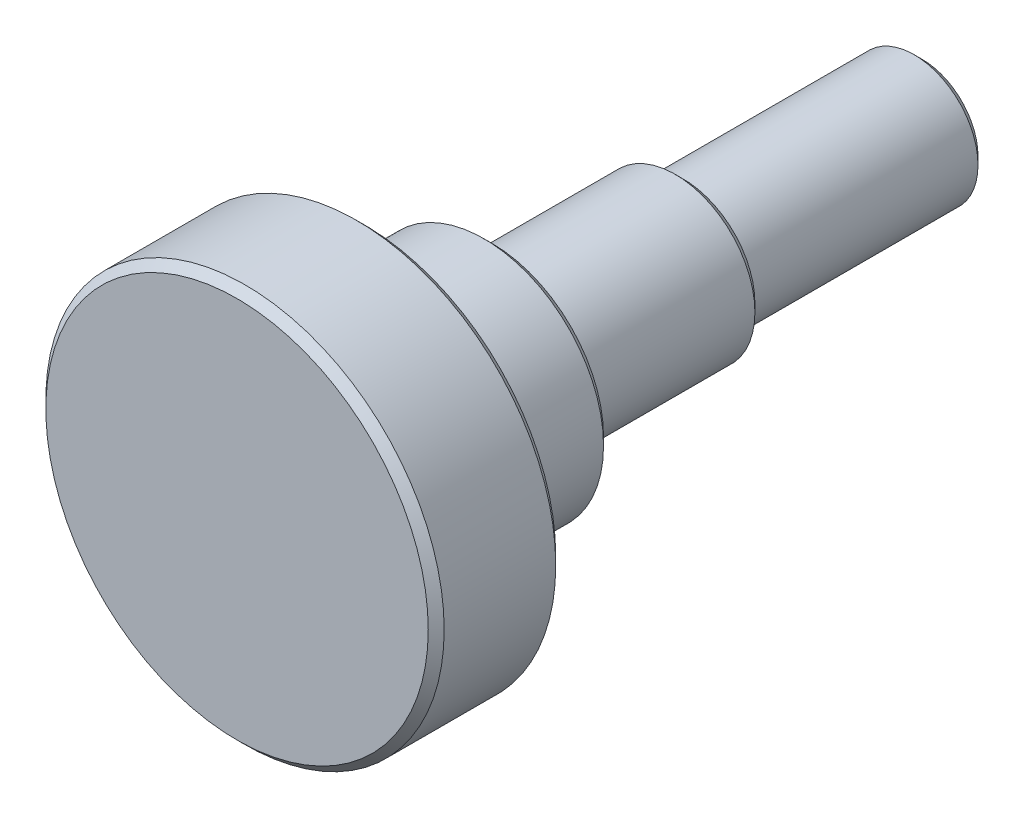
SolidWorks part; units mm, degrees
material "S45C"
ref_plane "Front Plane" through (0, 0, 0) normal (0, 0, 1) x (1, 0, 0)
ref_plane "Top Plane" through (0, 0, 0) normal (0, 1, 0) x (1, 0, 0)
ref_plane "Right Plane" through (0, 0, 0) normal (1, 0, 0) x (0, 0, -1)
sketch "Sketch1" plane through (0, 0, 0) normal (0, 0, 1) x (1, 0, 0)
  circle A0 centre (0, 0) radius 4
  dimension "D1" = 8
extrude "Boss-Extrude1" add sketch "Sketch1" along normal blind 15
cosmetic thread "Cosmetic Thread1" parameters "D2"=6.891
sketch "Sketch2" plane through (0, 0, 15) normal (0, 0, 1) x (1, 0, 0)
  circle A0 centre (0, 0) radius 5
  dimension "D1" = 10
extrude "Boss-Extrude2" add sketch "Sketch2" along normal blind 12
sketch "Sketch3" plane through (0, 0, 27) normal (0, 0, 1) x (1, 0, 0)
  circle A0 centre (0, 0) radius 7.5
  dimension "D1" = 15
extrude "Boss-Extrude3" add sketch "Sketch3" along normal blind 8
sketch "Sketch4" plane through (0, 0, 35) normal (0, 0, 1) x (1, 0, 0)
  circle A0 centre (0, 0) radius 12.5
  dimension "D1" = 25
extrude "Boss-Extrude4" add sketch "Sketch4" along normal blind 8
chamfer "Chamfer1" distance 0.5 angle 45 5 edges at (12.5, 0, 43) (12.5, 0, 35) (7.5, 0, 27) (5, 0, 15) (4, 0, 0)
